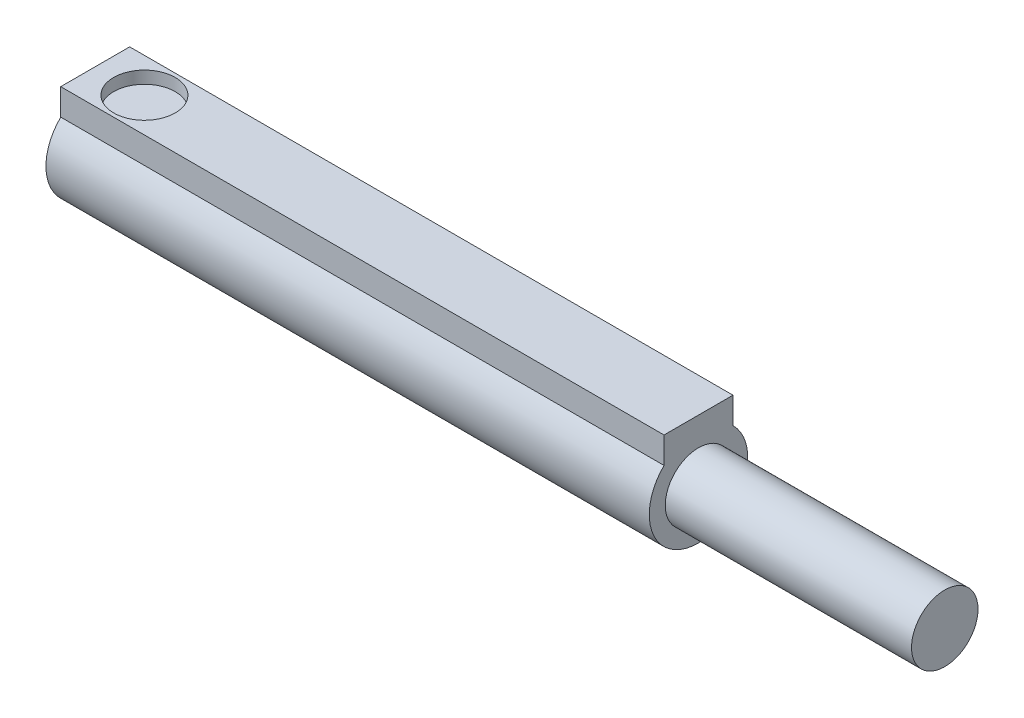
from build123d import *

# Parameters (mm, degrees)
BOSS_EXTRUDE1_DEPTH = 24.5
SKETCH2_R           = 1.35
BOSS_EXTRUDE2_DEPTH = 10
SKETCH3_R           = 1.25
CUT_EXTRUDE1_DEPTH  = 0.5


with BuildPart() as part:
    # Sketch1 → Boss-Extrude1 (new body)
    with BuildSketch(Plane(origin=(0, 0, 0), x_dir=(0, 0, -1), z_dir=(1, 0, 0))):
        with BuildLine():
            Line((1.4, 1.428285686), (1.4, 2.5))
            Line((1.4, 2.5), (-1.4, 2.5))
            Line((-1.4, 2.5), (-1.4, 1.428285686))
            ThreePointArc((-1.4, 1.428285686), (0, -2), (1.4, 1.428285686))
        make_face()
    extrude(amount=BOSS_EXTRUDE1_DEPTH)

    # Sketch2 → Boss-Extrude2 (add)
    with BuildSketch(Plane(origin=(24.5, 0, 0), x_dir=(0, 0, -1), z_dir=(1, 0, 0))):
        Circle(SKETCH2_R)
    extrude(amount=BOSS_EXTRUDE2_DEPTH)

    # Sketch3 → Cut-Extrude1 (cut)
    with BuildSketch(Plane(origin=(0, 2.5, 0), x_dir=(-1, 0, 0), z_dir=(0, 1, 0))):
        with Locations(Location((-2, 0, 0), (0, 0, 90))):
            Circle(SKETCH3_R)
    extrude(amount=-CUT_EXTRUDE1_DEPTH, mode=Mode.SUBTRACT)


solid = part.part
